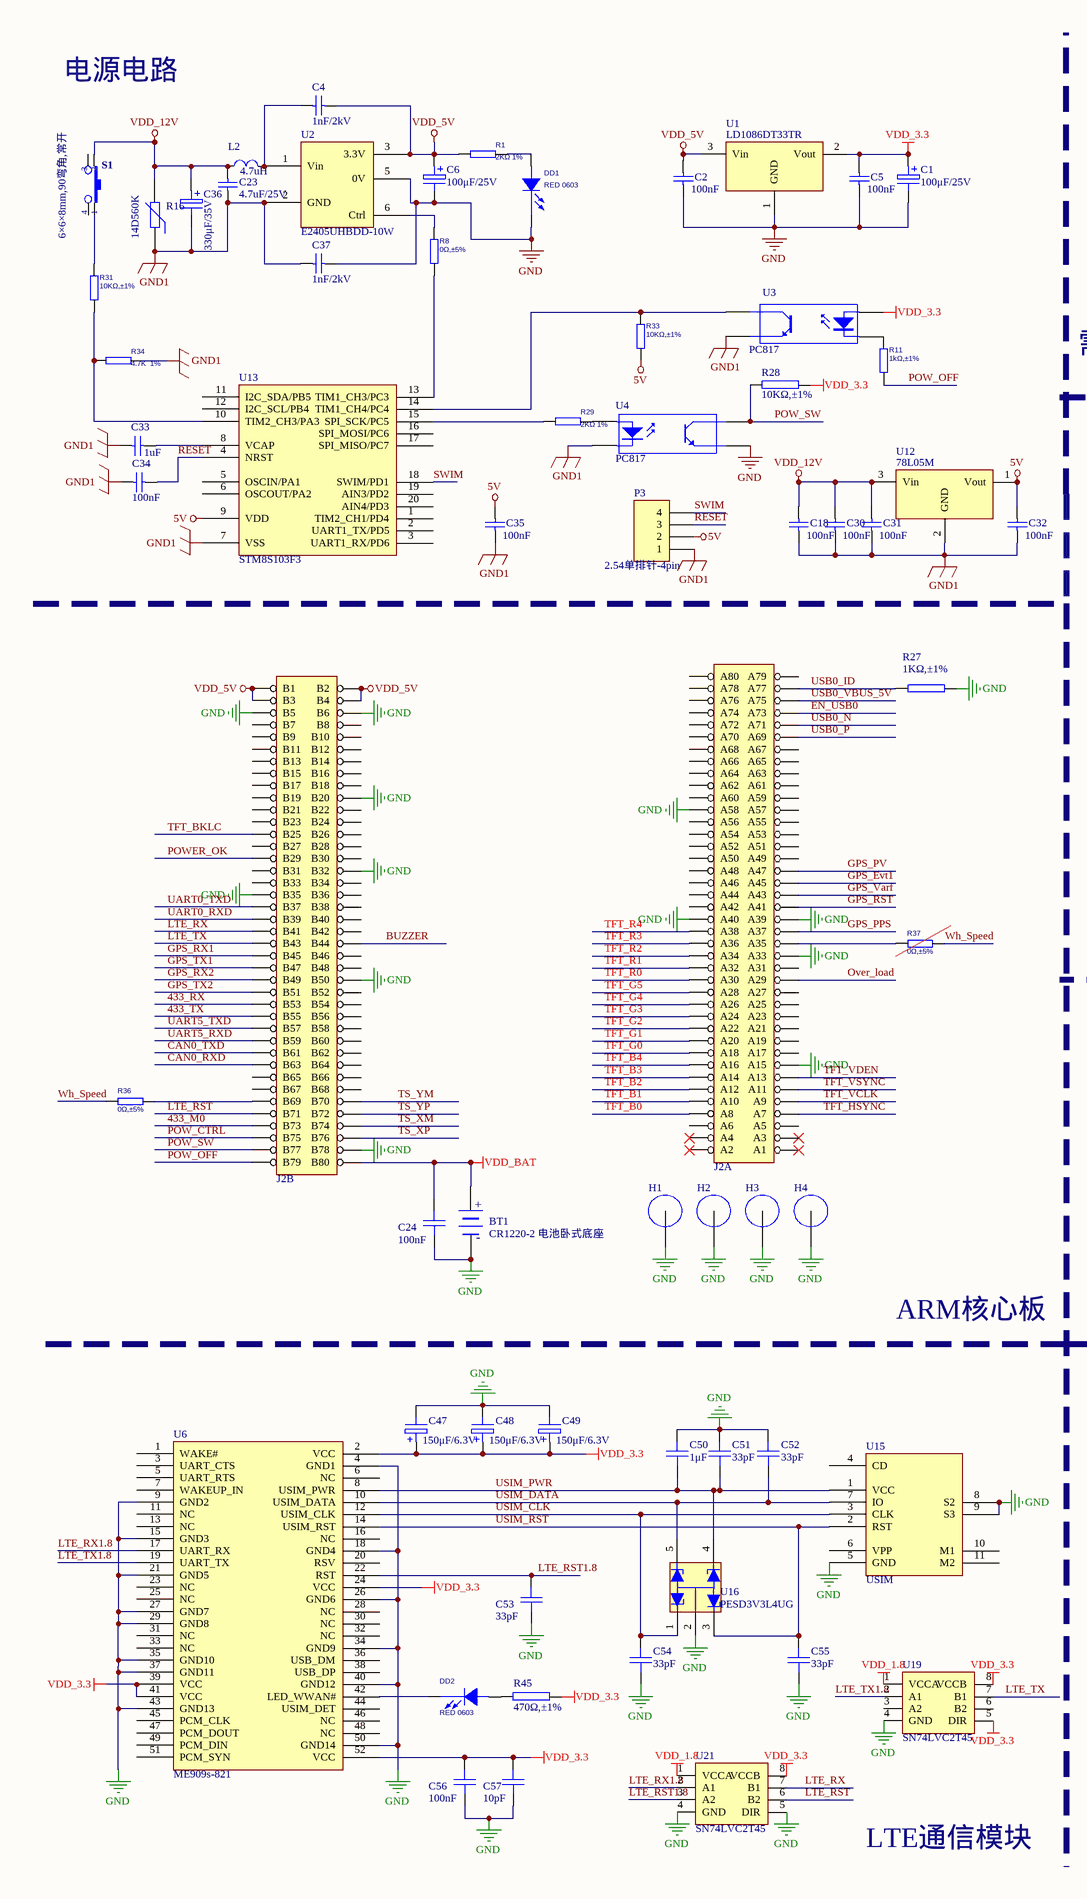
[diagram p0: MISC82794-3.SchDoc, left]
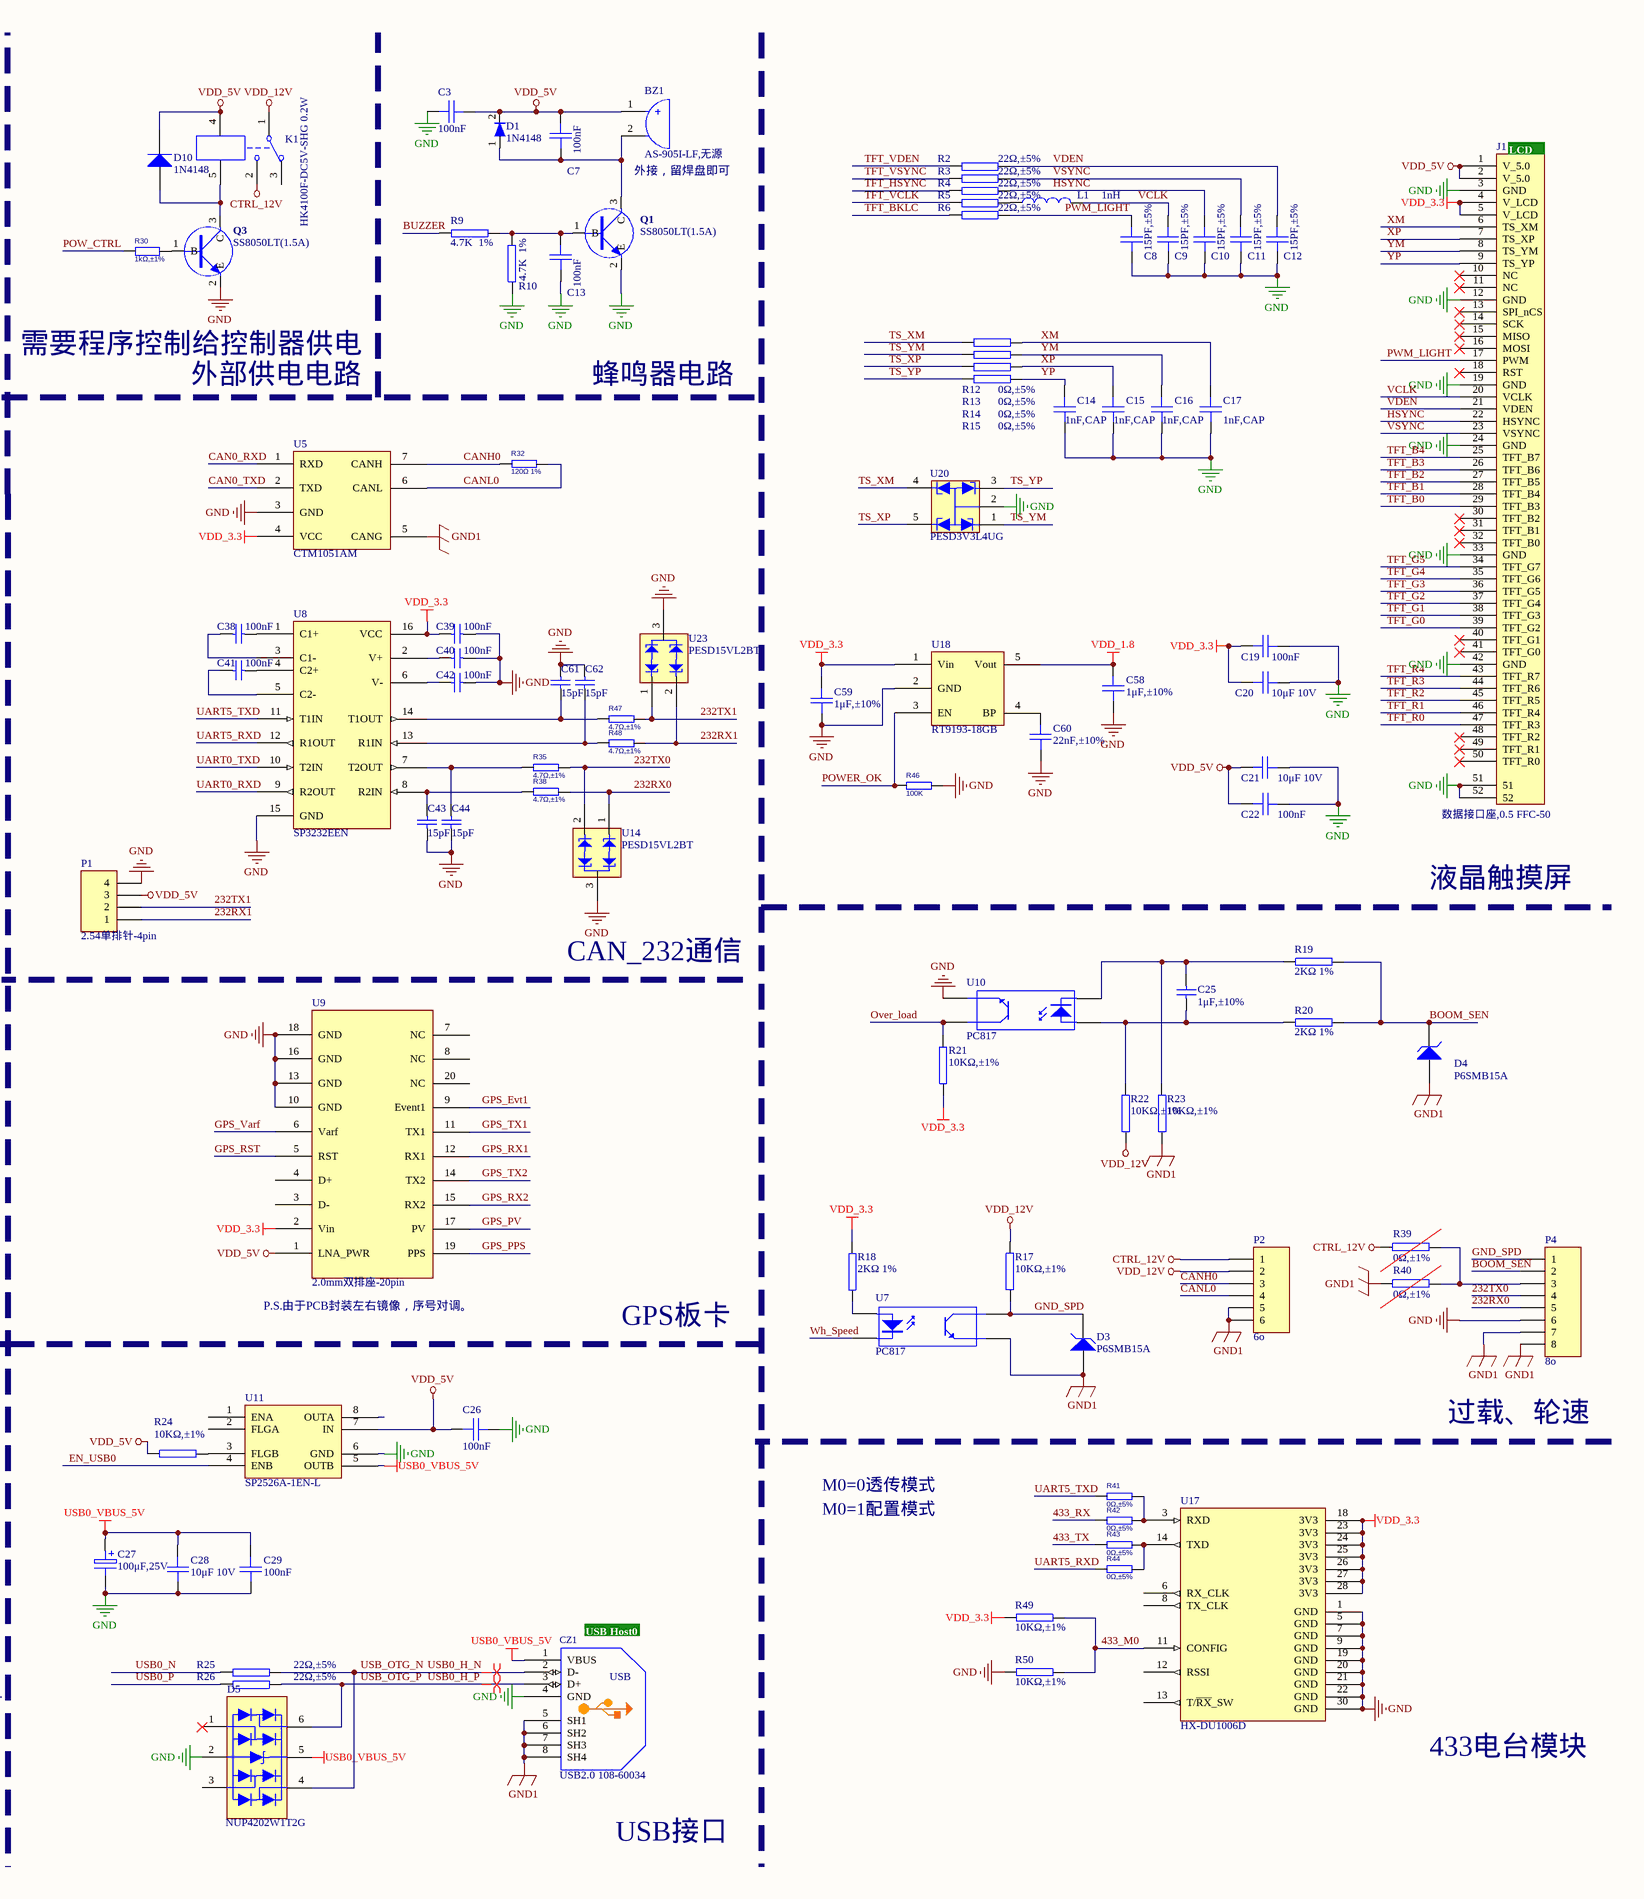
[diagram p1: MISC82794-3.SchDoc, right]
# Altium project MISC82794-4.PrjPcb
1 sheet, 157 parts. Net scope: global (net labels, ports and power ports of the same name join across sheets).
Board file: MISC82794.PcbDoc

## Sheet MISC82794-3.SchDoc
size A2

### Parts
BT1  value CR1220-2 电池卧式底座  [BATTERY-1220-1]  (hidden comment: BATTERY)
BZ1  value AS-905I-LF,无源  [XH2.5-2P]  (hidden comment: BUZZER2)
C1  100μF/25V  [RB6.3*7]
C2  100nF  [0805C]
C3  100nF  [0805C]
C4  1nF/2kV  [C1206]
C5  100nF  [0805C]
C6  100μF/25V  [RB6.3*7]
C7  100nF  [0805C]
C8  15PF,±5%  [0805C]
C9  15PF,±5%  [0805C]
C10  15PF,±5%  [0805C]
C11  15PF,±5%  [0805C]
C12  15PF,±5%  [0805C]
C13  100nF  [0805C]
C14  1nF,CAP  [0805C]
C15  1nF,CAP  [0805C]
C16  1nF,CAP  [0805C]
C17  1nF,CAP  [0805C]
C18  100nF  [0805C]
C19  100nF  [0805C]
C20  10μF 10V  [0805C]
C21  10μF 10V  [0805C]
C22  100nF  [0805C]
C23  4.7uF/25V  [C1206]
C24  100nF  [0805C]
C25  1μF,±10%  [0805C]
C26  100nF  [0805C]
C27  100μF,25V  [CAPPRD250W45D630H800P]
C28  10μF 10V  [0805C]
C29  100nF  [0805C]
C30  100nF  [0805C]
C31  100nF  [0805C]
C32  100nF  [0805C]
C33  1uF  [0805C]
C34  100nF  [0805C]
C35  100nF  [0805C]
C36  330μF/35V  [CAPPR5.0-10X16-0.8]
C37  1nF/2kV  [C1206]
C38  100nF  [0805C]
C39  100nF  [0805C]
C40  100nF  [0805C]
C41  100nF  [0805C]
C42  100nF  [0805C]
C43  15pF  [0805C]
C44  15pF  [0805C]
C47  150μF/6.3V  [CT3528-B]
C48  150μF/6.3V  [CT3528-B]
C49  150μF/6.3V  [CT3528-B]
C50  1μF  [0805C]
C51  33pF  [0805C]
C52  33pF  [0805C]
C53  33pF  [0805C]
C54  33pF  [0805C]
C55  33pF  [0805C]
C56  100nF  [0805C]
C57  10pF  [0805C]
C58  1μF,±10%  [0805C]
C59  1μF,±10%  [0805C]
C60  22nF,±10%  [0805C]
C61  15pF  [0805C]
C62  15pF  [0805C]
CZ1  value USB2.0 108-60034  [USB-1400]  (hidden comment: USB)
D1  1N4148  [SMD-D4148]
D3  P6SMB15A  [DO-214]
D4  P6SMB15A  [DO-214]
D5  value NUP4202W1T2G  [SOT-363]  (hidden comment: NUP4202W1)
D10  1N4148  [SMD-D4148]
DD1  RED 0603  [LED0805]
DD2  RED 0603  [LED0805]
H1  Hole  [HOLE-3.2]  (value not drawn)
H2  Hole  [HOLE-3.2]  (value not drawn)
H3  Hole  [HOLE-3.2]  (value not drawn)
H4  Hole  [HOLE-3.2]  (value not drawn)
J1  value 数据接口座,0.5 FFC-50  [FFC0.5-50P-A]  (hidden comment: FPC-50)
J2  HEADER 40X2  [AM3352B]  (value not drawn)  (parts A,B of 2)
K1  HK4100F-DC5V-SHG 0.2W  [HK4100F]
L1  1nH  [0805R]
L2  4.7uH  [SLF6045]
P1  2.54单排针-4pin  [HDR1X4]
P2  6о  [BBD-06PMFP-LC7001]
P3  2.54单排针-4pin  [HDR1X4]
P4  8о  [BDU-08PMFP-LC7001]
Q1  SS8050LT(1.5A)  [SOT-23]
Q3  SS8050LT(1.5A)  [SOT-23]
R1  2KΩ 1%  [0805R]
R2  22Ω,±5%  [0805R]
R3  22Ω,±5%  [0805R]
R4  22Ω,±5%  [0805R]
R5  22Ω,±5%  [0805R]
R6  22Ω,±5%  [0805R]
R8  0Ω,±5%  [0805R]
R9  4.7K  1%  [0805R]
R10  4.7K  1%  [0805R]
R11  1kΩ,±1%  [0805R]
R12  0Ω,±5%  [0805R]
R13  0Ω,±5%  [0805R]
R14  0Ω,±5%  [0805R]
R15  0Ω,±5%  [0805R]
R16  14D560K  [14D560K]
R17  10KΩ,±1%  [0805R]
R18  2KΩ 1%  [0805R]
R19  2KΩ 1%  [0805R]
R20  2KΩ 1%  [0805R]
R21  10KΩ,±1%  [0805R]
R22  10KΩ,±1%  [0805R]
R23  10KΩ,±1%  [0805R]
R24  10KΩ,±1%  [0805R]
R25  22Ω,±5%  [0805R]
R26  22Ω,±5%  [0805R]
R27  1KΩ,±1%  [0805R]
R28  10KΩ,±1%  [0805R]
R29  2KΩ 1%  [0805R]
R30  1kΩ,±1%  [0805R]
R31  10KΩ,±1%  [0805R]
R32  120Ω 1%  [0805R]
R33  10KΩ,±1%  [0805R]
R34  4.7K  1%  [0805R]
R35  4.7Ω,±1%  [0805R]
R36  0Ω,±5%  [0805R]
R37  0Ω,±5%  [0805R]
R38  4.7Ω,±1%  [0805R]
R39  0Ω,±1%  [0805R]
R40  0Ω,±1%  [0805R]
R41  0Ω,±5%  [0805R]
R42  0Ω,±5%  [0805R]
R43  0Ω,±5%  [0805R]
R44  0Ω,±5%  [0805R]
R45  470Ω,±1%  [0805R]
R46  100K  [0805R]
R47  4.7Ω,±1%  [0805R]
R48  4.7Ω,±1%  [0805R]
R49  10KΩ,±1%  [0805R]
R50  10KΩ,±1%  [0805R]
S1  value 6×6×8mm,90弯角,常开  [SWICH4.5]  (hidden comment: SW-PB4P)
U1  LD1086DT33TR  [DPAK]
U2  E2405UHBDD-10W  [E2403UHBDD]
U3  PC817  [SMD-4]
U4  PC817  [SMD-4]
U5  CTM1051AM  [CTM1051AM]
U6  ME909s-821
U7  PC817  [SMD-4]
U8  SP3232EEN  [SOP16-6.6]
U9  2.0mm双排座-20pin  [20PIN-OEM_STARA]
U10  PC817  [SMD-4]
U11  value SP2526A-1EN-L  [SOIC127P600X175-8N]  (hidden comment: SP2526A)
U12  78L05M  [SOT-89]
U13  STM8S103F3  [TSOP65P640X120-20N]
U14  PESD15VL2BT  [SOT-23]
U15  USIM
U16  PESD3V3L4UG  [SOT-353]
U17  HX-DU1006D  [HX-DU1006D]
U18  RT9193-18GB  [SOT23-5]
U19  SN74LVC2T45
U20  PESD3V3L4UG  [SOT-353]
U21  SN74LVC2T45
U23  PESD15VL2BT  [SOT-23]

### Nets
5V: C32.1 C35.1 P3.2 R33.1 U12.1(Vout) U13.9(VDD)
CTRL_12V: K1.2 P2.1 R39.2
GND: BT1.2(-) C1.2 C2.2 C3.2 C5.2 C6.2 C8.2 C9.2 C10.2 C11.2 C12.2 C13.1 C14.2 C15.2 C16.2 C17.2 C19.1 C20.1 C21.2 C22.1 C24.2 C26.1 C27.2 C28.2 C29.2 C37.2 C39.2 C40.2 C42.2 C43.2 C44.2 C47.2 C48.2 C49.2 C50.2 C51.2 C52.2 C53.2 C54.1 C55.1 C56.2 C57.2 C58.1 C59.1 C60.1 C61.1 C62.1 CZ1.4(GND) D5.2 DD1.2(ANODE) H1.8(CANH) H2.8(CANH) H3.8(CANH) H4.8(CANH) J1.3(GND) J1.12(GND) J1.19(GND) J1.24(GND) J1.33(GND) J1.42(GND) J1.51 J1.52 J2.A15 J2.A33 J2.A39 J2.A40 J2.A58 J2.B5 J2.B6 J2.B20 J2.B32 J2.B35 J2.B50 J2.B78 P1.4 P4.6 Q1.2(E) Q3.2(E) R10.1 R27.1 R46.2 R50.2 U1.1(GND) U2.5(0V) U4.3(E) U5.3(GND) U6.4(GND1) U6.9(GND2) U6.15(GND3) U6.18(GND4) U6.21(GND5) U6.26(GND6) U6.27(GND7) U6.29(GND8) U6.34(GND9) U6.35(GND10) U6.37(GND11) U6.40(GND12) U6.43(GND13) U6.50(GND14) U8.15(GND) U9.10(GND) U9.13(GND) U9.16(GND) U9.18(GND) U10.3(E) U11.6(GND) U14.3 U15.5(GND) U15.8(S2) U15.9(S3) U16.2 U17.1(GND) U17.5(GND) U17.7(GND) U17.9(GND) U17.19(GND) U17.20(GND) U17.21(GND) U17.22(GND) U17.30(GND) U18.2(GND) U19.4(GND) U20.2 U21.4(GND) U21.5(DIR) U23.3
GND1: C18.2 C23.1 C30.2 C31.2 C32.2 C33.1 C34.1 C35.2 C36.2 C37.1 CZ1.5(SH1) CZ1.6(SH2) CZ1.7(SH3) CZ1.8(SH4) D3.1(A) D4.1(A) P2.5 P2.6 P3.1 P4.7 P4.8 R16.1 R23.2 R34.1 R40.2 U2.2(GND) U3.3(E) U4.2(K) U5.5(CANG) U7.3(E) U12.2(GND) U13.7(VSS)
USB0_VBUS_5V: C27.1 C28.1 C29.1 CZ1.1(VBUS) D5.5 J2.A75 U11.5(OUTB)
VDD_1.8: C58.2 U18.5(Vout) U19.1(VCCA) U21.1(VCCA)
VDD_3.3: C1.1 C5.1 C19.2 C20.2 C39.1 C47.1 C48.1 C49.1 C56.1 C57.1 C59.2 J1.4(V_LCD) J1.5(V_LCD) R18.1 R21.1 R28.1 R45.1 R49.2 U1.2(Vout) U3.1(A) U5.4(VCC) U6.2(VCC) U6.24(VCC) U6.39(VCC) U6.41(VCC) U6.52(VCC) U8.16(VCC) U9.2(Vin) U17.18(3V3) U17.23(3V3) U17.24(3V3) U17.25(3V3) U17.26(3V3) U17.27(3V3) U17.28(3V3) U18.1(Vin) U19.5(DIR) U19.8(VCCB) U21.8(VCCB)
VDD_5V: BZ1.1(A) C2.1 C3.1 C4.2 C6.1 C7.2 C21.1 C22.2 C26.2 D1.2 D10.2(K) J1.1(V_5.0) J1.2(V_5.0) J2.B1 J2.B2 J2.B3 J2.B4 K1.4 P1.3 R1.2 R24.2 U1.3(Vin) U2.3(3.3V) U9.1(LNA_PWR) U11.7(IN)
VDD_12V: C18.1 C23.2 C30.1 C31.1 C36.1 K1.1 L2.1 P2.2 R16.2 R17.2 R22.2 S1.2 U12.3(Vin)
VDD_BAT: BT1.1(+) C24.1 J2.B80
232RX0: P4.5 R38.1 U14.1
232RX1: P1.1 R48.1 U23.2
232TX0: P4.4 R35.1 U14.2
232TX1: P1.2 R47.1 U23.1
433_M0: J2.B73 R49.1 R50.1 U17.11(CONFIG)
433_RX: J2.B53 R42.1
433_TX: J2.B55 R43.1
BOOM_SEN: D4.2(K) P4.2 R19.1 R20.1
BUZZER: J2.B44 R9.1
CAN0_RXD: J2.B63 U5.1(RXD)
CAN0_TXD: J2.B61 U5.2(TXD)
CANH0: P2.3 R32.1 U5.7(CANH)
CANL0: P2.4 R32.2 U5.6(CANL)
EN_USB0: J2.A73 U11.4(ENB)
GND_SPD: D3.2(K) P4.1 R17.1 U7.4(C)
GPS_Evt1: J2.A45 U9.9(Event1)
GPS_PPS: J2.A37 U9.19(PPS)
GPS_PV: J2.A47 U9.17(PV)
GPS_RST: J2.A41 U9.5(RST)
GPS_RX1: J2.B45 U9.12(RX1)
GPS_RX2: J2.B49 U9.15(RX2)
GPS_TX1: J2.B47 U9.11(TX1)
GPS_TX2: J2.B51 U9.14(TX2)
GPS_Varf: J2.A43 U9.6(Varf)
HSYNC: C10.1 J1.22(HSYNC) R4.2
LTE_RST: J2.B71 U21.6(B2)
LTE_RST1.8: C53.1 U6.22(RST) U21.3(A2)
LTE_RX: J2.B41 U21.7(B1)
LTE_RX1.8: U6.17(UART_RX) U21.2(A1)
LTE_TX: J2.B43 U19.7(B1)
LTE_TX1.8: U6.19(UART_TX) U19.2(A1)
Over_load: J2.A29 R21.2 U10.4(C)
POW_CTRL: J2.B75 R30.1
POW_OFF: J2.B79 R11.1
POW_SW: J2.B77 R28.2 U4.4(C)
POWER_OK: J2.B29 R46.1 U18.3(EN)
PWM_LIGHT: C8.1 J1.17(PWM) R6.2
RESET: C34.2 P3.3 U13.4(NRST)
SWIM: P3.4 U13.18(SWIM/PD1)
TFT_B0: J1.29(TFT_B3) J2.A8
TFT_B1: J1.28(TFT_B4) J2.A10
TFT_B2: J1.27(TFT_B5) J2.A12
TFT_B3: J1.26(TFT_B6) J2.A14
TFT_B4: J1.25(TFT_B7) J2.A16
TFT_BKLC: J2.B25 R6.1
TFT_G0: J1.39(TFT_G2) J2.A18
TFT_G1: J1.38(TFT_G3) J2.A20
TFT_G2: J1.37(TFT_G4) J2.A22
TFT_G3: J1.36(TFT_G5) J2.A24
TFT_G4: J1.35(TFT_G6) J2.A26
TFT_G5: J1.34(TFT_G7) J2.A28
TFT_HSYNC: J2.A7 R4.1
TFT_R0: J1.47(TFT_R3) J2.A30
TFT_R1: J1.46(TFT_R4) J2.A32
TFT_R2: J1.45(TFT_R5) J2.A34
TFT_R3: J1.44(TFT_R6) J2.A36
TFT_R4: J1.43(TFT_R7) J2.A38
TFT_VCLK: J2.A9 R5.1
TFT_VDEN: J2.A13 R2.1
TFT_VSYNC: J2.A11 R3.1
TS_XM: J2.B74 R12.1 U20.4
TS_XP: J2.B76 R14.1 U20.5
TS_YM: J2.B70 R13.1 U20.1
TS_YP: J2.B72 R15.1 U20.3
UART0_RXD: J2.B39 U8.9(R2OUT)
UART0_TXD: J2.B37 U8.10(T2IN)
UART5_RXD: J2.B59 R44.1 U8.12(R1OUT)
UART5_TXD: J2.B57 R41.1 U8.11(T1IN)
USB0_H_N: CZ1.2(D-) D5.4 R25.2  [also labelled USB_OTG_N]
USB0_H_P: CZ1.3(D+) D5.6 R26.2  [also labelled USB_OTG_P]
USB0_ID: J2.A77 R27.2
USB0_N: J2.A71 R25.1
USB0_P: J2.A69 R26.1
USIM_CLK: C54.2 U6.12(USIM_CLK) U15.3(CLK) U16.1
USIM_DATA: C52.1 U6.10(USIM_DATA) U15.7(IO) U16.5
USIM_PWR: C50.1 C51.1 U6.8(USIM_PWR) U15.1(VCC) U16.4
USIM_RST: C55.2 U6.14(USIM_RST) U15.2(RST) U16.3
VCLK: C9.1 J1.20(VCLK) L1.2
VDEN: C12.1 J1.21(VDEN) R2.2
VSYNC: C11.1 J1.23(VSYNC) R3.2
Wh_Speed: R36.1 R37.1 U7.2(K)
XM: C17.1 J1.6(TS_XM) R12.2
XP: C15.1 J1.7(TS_XP) R14.2
YM: C16.1 J1.8(TS_YM) R13.2
YP: C14.1 J1.9(TS_YP) R15.2
NetBZ1_2: BZ1.2(B) C7.1 D1.1 Q1.3(C)
NetC4_1: C4.1 L2.2 U2.1(Vin)
NetC13_2: C13.2 Q1.1(B) R9.2 R10.2
NetC25_1: C25.1 R20.2 R22.1 U10.1(A)
NetC25_2: C25.2 R19.2 R23.1 U10.2(K)
NetC33_2: C33.2 U13.8(VCAP)
NetC38_1: C38.1 U8.3(C1-)
NetC38_2: C38.2 U8.1(C1+)
NetC40_1: C40.1 U8.2(V+)
NetC41_1: C41.1 U8.5(C2-)
NetC41_2: C41.2 U8.4(C2+)
NetC42_1: C42.1 U8.6(V-)
NetC43_1: C43.1 R38.2 U8.8(R2IN)
NetC44_1: C44.1 R35.2 U8.7(T2OUT)
NetC60_2: C60.2 U18.4(BP)
NetC61_2: C61.2 R47.2 U8.14(T1OUT)
NetC62_2: C62.2 R48.2 U8.13(R1IN)
NetD10_1: D10.1(A) K1.5 Q3.3(C)
NetDD1_1: DD1.1(CATHODE) R1.1
NetDD2_1: DD2.1(CATHODE) R45.2
NetDD2_2: DD2.2(ANODE) U6.42(LED_WWAN#)
NetJ2_A35: J2.A35 R37.2
NetJ2_B69: J2.B69 R36.2
NetL1_1: L1.1 R5.2
NetP4_3: P4.3 R39.1 R40.1
NetQ3_1: Q3.1(B) R30.2
NetR8_1: R8.1 U2.6(Ctrl)
NetR8_2: R8.2 U13.13(TIM1_CH3/PC3)
NetR11_2: R11.2 U3.2(K)
NetR18_2: R18.2 U7.1(A)
NetR24_1: R24.1 U11.3(FLGB)
NetR29_1: R29.1 U4.1(A)
NetR29_2: R29.2 U13.15(SPI_SCK/PC5)
NetR31_1: R31.1 S1.1
NetR31_2: R31.2 R34.2 U13.10(TIM2_CH3/PA3)
NetR33_2: R33.2 U3.4(C) U13.14(TIM1_CH4/PC4)
NetR41_2: R41.2 R42.2 U17.3(RXD)
NetR43_2: R43.2 R44.2 U17.14(TXD)

Not connected (* = marked no-connect by the designer): D5 1* 3; J1 10(NC)* 11(NC)* 13(SPI_nCS)* 14(SCK)* 15(MISO)* 16(MOSI)* 18(RST)* 30(TFT_B2)* 31(TFT_B1)* 32(TFT_B0)* 40(TFT_G1)* 41(TFT_G0)* 48(TFT_R2)* 49(TFT_R1)* 50(TFT_R0)*; J2 A1* A2* A3* A4* A5 A6 A17 A19 A21 A23 A25 A27 A31 A42 A44 A46 A48 A49 A50 A51 A52 A53 A54 A55 A56 A57 A59 A60 A61 A62 A63 A64 A65 A66 A67 A68 A70 A72 A74 A76 A78 A79 A80 B7 B8 B9 B10 B11 B12 B13 B14 B15 B16 B17 B18 B19 B21 B22 B23 B24 B26 B27 B28 B30 B31 B33 B34 B36 B38 B40 B42 B46 B48 B52 B54 B56 B58 B60 B62 B64 B65 B66 B67 B68; K1 3(2); S1 3 4; U6 1(WAKE#) 3(UART_CTS) 5(UART_RTS) 6(NC) 7(WAKEUP_IN) 11(NC) 13(NC) 16(NC) 20(RSV) 23(NC) 25(NC) 28(NC) 30(NC) 31(NC) 32(NC) 33(NC) 36(USB_DM) 38(USB_DP) 44(USIM_DET) 45(PCM_CLK) 46(NC) 47(PCM_DOUT) 48(NC) 49(PCM_DIN) 51(PCM_SYN); U9 3(D-) 4(D+) 7(NC) 8(NC) 20(NC); U11 1(ENA) 2(FLGA) 8(OUTA); U13 1(TIM2_CH1/PD4) 2(UART1_TX/PD5) 3(UART1_RX/PD6) 5(OSCIN/PA1) 6(OSCOUT/PA2) 11(I2C_SDA/PB5) 12(I2C_SCL/PB4) 16(SPI_MOSI/PC6) 17(SPI_MISO/PC7) 19(AIN3/PD2) 20(AIN4/PD3); U15 4(CD) 6(VPP) 10(M1) 11(M2); U17 6(RX_CLK) 8(TX_CLK) 12(RSSI) 13(T/~{RX}_SW); U19 3(A2) 6(B2)

### Layout directives
differential pair: USB0_H_N, USB0_H_P

### Notes on the sheet
- 电源电路
- (near J1) LCD
- 外接，留焊盘即可
- 需要程序控制给控制器供电
- 外部供电电路
- 蜂鸣器电路
- 液晶触摸屏
- CAN_232通信
- ARM核心板
- (near U9) P.S.由于PCB封装左右镜像，序号对调。
- GPS板卡
- 过载、轮速
- M0=0透传模式
- M0=1配置模式
- (near CZ1) USB Host0
- 433电台模块
- LTE通信模块
- USB接口

### Library data of the parts
BT1 = 1.10.05.0096: 2P,间距1.25mm,Wafer凹槽边框,90°,FPC2-49T; 名称: 插座; 贴片和直插: SMT; 物料代码: 1.10.05.0096; 封装: FPC2-49T; 型号: 2P,间距1.25mm,Wafer凹槽边框,90°; ComponentLink1Description: ErpDataInfo
BZ1 = 1.06.09.0016: AS-905I-LF,无源,Ф9×4.8mm,常州立翔,RoHS; 名称: 讯响器; 厂商: 常州笠翔; 贴片和直插: THT; PCB备注: Flq-Shcj-Twrj-150113; 器件优选方案: 量产物料,优先选用; 物料代码: 1.06.09.0016; RoHS: RoHS; 型号: AS-905I-LF,无源,Ф9×4.8mm; ComponentLink1Description: ErpDataInfo
C1 C6 C27 C36 C47-C49 = 1.02.11.0018: 220μF,16V,Ф6.3×7mm,,珠海华冠,RoHS; 名称: 电解电容; 贴片和直插: THT; 器件优选方案: 状态正常; PCB备注: Fcqh-Slq-Twrj-141216; 物料代码: 1.02.11.0018; 厂商: 珠海华冠; RoHS: RoHS; 型号: 220μF,16V,Ф6.3×7mm; ComponentLink1Description: ErpDataInfo
  C1 C6: Value: 100μF/25V
  C27: Value: 100μF,25V
  C36: Value: 330μF/35V
  C47-C49: Value: 150μF/6.3V
C2 C4 C5 C18 C23 C30-C35 C37 = Cap Semi: Capacitor (Semiconductor SIM Model); Published: 8-Jun-2000; Revision: July-2002: Re-released for DXP Platform.; Publisher: Altium Limited
  C2 C5 C18 C30-C32 C34 C35: Value: 100nF
  C4 C37: Value: 1nF/2kV
  C23: Value: 4.7uF/25V
  C33: Value: 1uF
C3 C7 C13 C19 C22 C24 C26 C50-C57 = 1.02.17.0020: 0.1μF,±10%,X5R,25V,0402,RoHS; 名称: 电容; 封装: 0402; 设备封装名称: C0402_0.1uF_X5R_25V_10%; 贴片和直插: SMT; 物料代码: 1.02.17.0020; RoHS: RoHS; 型号: 0.1μF,±10%,X5R,25V; ComponentLink1Description: ErpDataInfo
  C3 C7 C13 C19 C22 C24 C26 C56: Value: 100nF
  C50: Value: 1μF
  C51-C55: Value: 33pF
  C57: Value: 10pF
C8-C12 = 1.02.17.0005: 15PF,±5%,50V,COG,0402,RoHS; 名称: 电容; 封装: 0402; 设备封装名称: C0402_15PF_COG_50V_5%; 贴片和直插: SMT; 物料代码: 1.02.17.0005; Value: 15PF,±5%; ComponentLink1Description: ErpDataInfo; RoHS: RoHS; 型号: 15PF,±5%,50V,COG
C14-C17 = 1.02.17.0021: 1nF,CAP,CER,1000PF,50V,CDG,GRM1555C1H102JA01D,0402,MURATA,RoHS; 名称: 电容; 封装: 0402; 贴片和直插: SMT; 物料代码: 1.02.17.0021; Value: 1nF,CAP; RoHS: RoHS; 型号: 1nF,CAP,CER,1000PF,50V,CDG,GRM1555C1H102JA01D; ComponentLink1Description: ErpDataInfo; 厂商: MURATA
C20 = 1.02.01.0065: 10uF,6.3V,X5R,GRM188R60J106ME47D,0603,Murata,RoHS; 名称: 电容; 封装: 0603; 贴片和直插: SMT; 物料代码: 1.02.01.0065; Value: 10μF 10V; 厂商: Murata; RoHS: RoHS; 型号: 10uF,6.3V,X5R,GRM188R60J106ME47D; ComponentLink1Description: ErpDataInfo
C21 = 1.02.02.0055: 106,10μF,±10%,10V,X5R,0805,RoHS; 名称: 电容; 封装: 0805; 设备封装名称: C0805_106_X5R_10V_10%; 贴片和直插: SMT; 物料代码: 1.02.02.0055; Value: 10μF 10V; RoHS: RoHS; 型号: 106,10μF,±10%,10V,X5R; ComponentLink1Description: ErpDataInfo
C25 = Cap: Capacitor; Value: 10nF; Published: 8-Jun-2000; Revision: July-2002: Re-released for DXP Platform.; Publisher: Altium Limited
C28 = 1.02.02.0055: 106,10μF,±10%,10V,X5R,0805,RoHS; 名称: 电容; 封装: 0805; 设备封装名称: C0805_106_X5R_10V_10%; 贴片和直插: SMT; 器件优选方案: 量产物料,优先选用; 物料代码: 1.02.02.0055; Value: 10μF 10V; RoHS: RoHS; 型号: 106,10μF,±10%,10V,X5R; ComponentLink1Description: ErpDataInfo
C29 = 1.02.17.0020: 0.1μF,±10%,X5R,25V,0402,RoHS; 名称: 电容; 封装: 0402; 设备封装名称: C0402_0.1uF_X5R_25V_10%; 贴片和直插: SMT; 器件优选方案: 状态正常; 物料代码: 1.02.17.0020; Value: 100nF; RoHS: RoHS; 型号: 0.1μF,±10%,X5R,25V; ComponentLink1Description: ErpDataInfo
C38-C44 C61 C62 = Cap: Capacitor; Published: 8-Jun-2000; Revision: July-2002: Re-released for DXP Platform.; Publisher: Altium Limited
  C38-C42: Value: 100nF
  C43 C44 C61 C62: Value: 15pF
C58 C59 = 1.02.17.0020: 1uF,±10%,X7R,25V; 名称: 电容; 封装: 0402; 设备封装名称: C0402_0.1uF_X5R_25V_10%; 贴片和直插: SMT; 型号: 0.1μF,±10%,X5R,25V; 物料代码: 1.02.17.0020; Value: 1μF,±10%; RoHS: RoHS; ComponentLink1Description: ErpDataInfo
C60 = 1.02.17.0020: 22nF,±10%,X5R,50V; 名称: 电容; 封装: 0402; 设备封装名称: C0402_0.1uF_X5R_25V_10%; 贴片和直插: SMT; 型号: 0.1μF,±10%,X5R,25V; 物料代码: 1.02.17.0020; Value: 22nF,±10%; RoHS: RoHS; ComponentLink1Description: ErpDataInfo
CZ1 = 1.10.12.0012: 3190004-H73-R,USB-A插座,立式,90°,THT,WCON,RoHS; Text Field1: 50; Text Field2: 60; 名称: USB插座(临时); 物料代码: 1.10.12.0012; 封装: THT; 厂商: WCON; RoHS: RoHS; 型号: 3190004-H73-R,USB-A插座,立式,90°; 贴片和直插: THT; ComponentLink1Description: ErpDataInfo
D1 = 1.04.07.0027: 1N4148,SOD-323,RoHS; 名称: 二极管; 设备封装名称: SOD-323_1N4148; 贴片和直插: SMT; 物料代码: 1.04.07.0027; Value: 1N4148; 封装: SOD-323; RoHS: RoHS; 型号: 1N4148; ComponentLink1Description: ErpDataInfo
D3 D4 = D Zener: Zener Diode; Published: 8-Jun-2000; LatestRevisionDate: 17-Jul-2002; LatestRevisionNote: Re-released for DXP Platform.; PackageReference: DIODE-0.7; Publisher: Altium Limited
D5 = 1.05.10.0376: NUP4202W1T2G,SC-88,ON,RoHS; 名称: IC; 贴片和直插: SMT; 物料代码: 1.05.10.0376; 封装: SC-88; 厂商: ON; RoHS: RoHS; 型号: NUP4202W1T2G; ComponentLink1Description: ErpDataInfo; 器件优选方案: *
D10 = Diode: Default Diode; Published: 8-Jun-2000; LatestRevisionDate: 17-Jul-2002; LatestRevisionNote: Re-released for DXP Platform.; PackageVersion: Sep-1996; PackageReference: SMC; PackageDescription: DO-214-AB/SMC; 2 C-Bend Leads; Body 7.9 x 5.9 mm, inc. leads (LxW); Code_JEDEC: DO-214-AB; Publisher: Altium Limited
DD1 DD2 = LED_0
J1 = 1.10.01.0028: 数据接口座,0.5FFC-50,SMD,下接,RoHS; 名称: 连接器-SMD; 贴片和直插: SMT; 物料代码: 1.10.01.0028; RoHS: RoHS; 型号: 数据接口座,0.5FFC-50,SMD,下接; ComponentLink1Description: ErpDataInfo
J2 = HEADER 40X2: DF12D(3.0)-80DP-0.5V(81),Fmale,SMT,HRS,RoHS; 物料代码: 1.10.14.0010; 名称: 板对板连接器(临时); PCB备注: 151026lmd; 器件优选方案: 样品物料,谨慎选用; 封装: SMT; 厂商: HRS; RoHS: RoHS; 型号: DF12D(3.0)-80DP-0.5V(81); 贴片和直插: SMT; ComponentLink1Description: ErpDataInfo
K1 = Relay-SPDT: Single-Pole Dual-Throw Relay; Published: 24-Mar-1999; LatestRevisionDate: 17-Jul-2002; LatestRevisionNote: Re-released for DXP Platform.; PackageReference: MODULE5B; Publisher: Altium Limited
L1 = 1.03.03.0022: BM02Y190S40R,0402,丰晶,RoHS; 名称: 磁珠; 封装: 0402; 贴片和直插: SMT; 物料代码: 1.03.03.0022; Value: 1nH; RoHS: RoHS; 型号: BM02Y190S40R; ComponentLink1Description: ErpDataInfo; 厂商: 丰晶
L2 = Inductor: Code_IEC: 1005; Published: 8-Jun-2000; LatestRevisionDate: 29-May-2009; LatestRevisionNote: IPC-7351 Footprint Added.; PackageReference: 0402-A; PackageDescription: Chip Inductor; Code_JEITA: 0402; Value: 4.7uH; Publisher: Altium Limited
P1 P3 = Header 4: Header, 4-Pin; LatestRevisionDate: 17-Jul-2002; LatestRevisionNote: Re-released for DXP Platform.; Publisher: Altium Limited
P2 = Header 6: Header, 6-Pin; LatestRevisionDate: 17-Jul-2002; LatestRevisionNote: Re-released for DXP Platform.; Publisher: Altium Limited
P4 = Header 8: Header, 8-Pin; LatestRevisionDate: 17-Jul-2002; LatestRevisionNote: Re-released for DXP Platform.; Publisher: Altium Limited
Q1 Q3 = 1.04.09.0001: SS8050LT(1.5A),SOT-23,江苏长电,RoHS; 名称: 三极管; 设备封装名称: SOT-23_SS8050LT; 贴片和直插: SMT; 物料代码: 1.04.09.0001; Value: SS8050LT(1.5A); 封装: SOT-23; 厂商: 江苏长电; RoHS: RoHS; 型号: SS8050LT(1.5A); ComponentLink1Description: ErpDataInfo
R1 R8 R11 R29-R38 R41-R44 R46-R48 = RES
  R1 R29: Value: 2KΩ 1%
  R8 R36 R37 R41-R44: Value: 0Ω,±5%
  R11 R30: Value: 1kΩ,±1%
  R31 R33: Value: 10KΩ,±1%
  R32: Value: 120Ω 1%
  R34: Value: 4.7K  1%
  R35 R38 R47 R48: Value: 4.7Ω,±1%
R2-R6 R25 R26 = 1.01.17.0023: 22Ω,±5%,0402,RALEC,RoHS; 名称: 电阻; 封装: 0402; 设备封装名称: R0402_22R; 贴片和直插: SMT; 物料代码: 1.01.17.0023; Value: 22Ω,±5%; RoHS: RoHS; 型号: 22Ω,±5%; ComponentLink1Description: ErpDataInfo; 厂商: RALEC
R9 R10 = 1.01.17.0019: 名称: 电阻; 规格型号: 4.7K,±5%,0402,RALEC,RoHS; 封装: 0402; 设备封装名称: R0402_4.7K; 厂商: RALEC; 贴片和直插: SMT; 物料代码: 1.01.17.0019; Value: 4.7K  1%; RoHS: RoHS; ComponentLink1Description: ErpDataInfo
R12-R15 = 1.01.17.0004: 0Ω,±5%,0402,RALEC,RoHS; 名称: 电阻; 封装: 0402; 设备封装名称: R0402_0R; 贴片和直插: SMT; 物料代码: 1.01.17.0004; Value: 0Ω,±5%; RoHS: RoHS; 型号: 0Ω,±5%; ComponentLink1Description: ErpDataInfo; 厂商: RALEC
R16 = Res Varistor: Varistor (Voltage-Sensitive Resistor); Published: 24-Mar-1999; LatestRevisionDate: 29-May-2009; LatestRevisionNote: IPC-7351 Footprint Added.; PackageVersion: Mar-2003; PackageReference: 6-0805; PackageDescription: Chip Resistor 0805 Case Size; Code_IPC: RESC2012; Publisher: Altium Limited
R17 R18 R28 R49 R50 = 1.01.17.0004: 名称: 电阻; 封装: 0402; 设备封装名称: R0402_0R; 型号: 0Ω,±5%; 贴片和直插: SMT; 厂商: RALEC; 物料代码: 1.01.17.0004; RoHS: RoHS; ComponentLink1Description: ErpDataInfo
  R17 R28 R49 R50: Value: 10KΩ,±1%
  R18: Value: 2KΩ 1%
R19 R20 = 1.01.17.0004: 名称: 电阻; 封装: 0402; 设备封装名称: R0402_0R; 型号: 1kΩ,±1%; 贴片和直插: SMT; 厂商: RALEC; 物料代码: 1.01.17.0004; Value: 2KΩ 1%; RoHS: RoHS; ComponentLink1Description: ErpDataInfo
R21 = 1.01.17.0004: 名称: 电阻; 封装: 0402; 设备封装名称: R0402_0R; 型号: 0Ω,±1%; 贴片和直插: SMT; 厂商: RALEC; 物料代码: 1.01.17.0004; Value: 10KΩ,±1%; RoHS: RoHS; ComponentLink1Description: ErpDataInfo
R22 R23 = 1.01.17.0004: 名称: 电阻; 封装: 0402; 设备封装名称: R0402_0R; 贴片和直插: SMT; 厂商: RALEC; 物料代码: 1.01.17.0004; Value: 10KΩ,±1%; RoHS: RoHS; ComponentLink1Description: ErpDataInfo
R24 R27 R39 R40 R45 = 1.01.17.0006: 10K,±5%,0402,RALEC,RoHS; 名称: 电阻; 封装: 0402; 设备封装名称: R0402_10K; 贴片和直插: SMT; 型号: 10K,±5%; 物料代码: 1.01.17.0006; RoHS: RoHS; ComponentLink1Description: ErpDataInfo; 厂商: RALEC
  R24: Value: 10KΩ,±1%
  R27: Value: 1KΩ,±1%
  R39 R40: Value: 0Ω,±1%
  R45: Value: 470Ω,±1%
S1 = SW-PB4P: 6×6×5.0mm,黑色,SMD,,*; 物料代码: 1.09.01.0003; 名称: 轻触按键; 贴片和直插: SMT; 型号: 6×6×5.0mm,黑色,SMD; ComponentLink1Description: ErpDataInfo
U1 U12 = VOLTREG1
U2 = E2403UHBDD-10W
U3 U4 U7 U10 = TLP281-1: Optoisolator
U8 = SP202ECT
U9 = OEMStar
U11 = 1.05.09.0064: 名称: IC; 规格型号: SP2526A-1EN-L,SO-8,Sipex,RoHS; 封装: SO-8; 设备封装名称: SO-8_SP2526A-1EN-L; 厂商: Sipex; 贴片和直插: SMT; 物料代码: 1.05.09.0064; RoHS: RoHS; ComponentLink1Description: ErpDataInfo; 型号: SP2526A-1EN-L
U14 U23 = PESD12VL2BT
U16 U20 = 1.05.10.0265: PESD3V3L4UG,SOT-353,NXP,RoHS; 名称: IC; 设备封装名称: SOT-353_PESD3V3L4UG; 贴片和直插: SMT; 物料代码: 1.05.10.0265; Value: PESD3V3L4UG; 封装: SOT-353; 厂商: NXP; RoHS: RoHS; 型号: PESD3V3L4UG; ComponentLink1Description: ErpDataInfo
U18 = RT9193